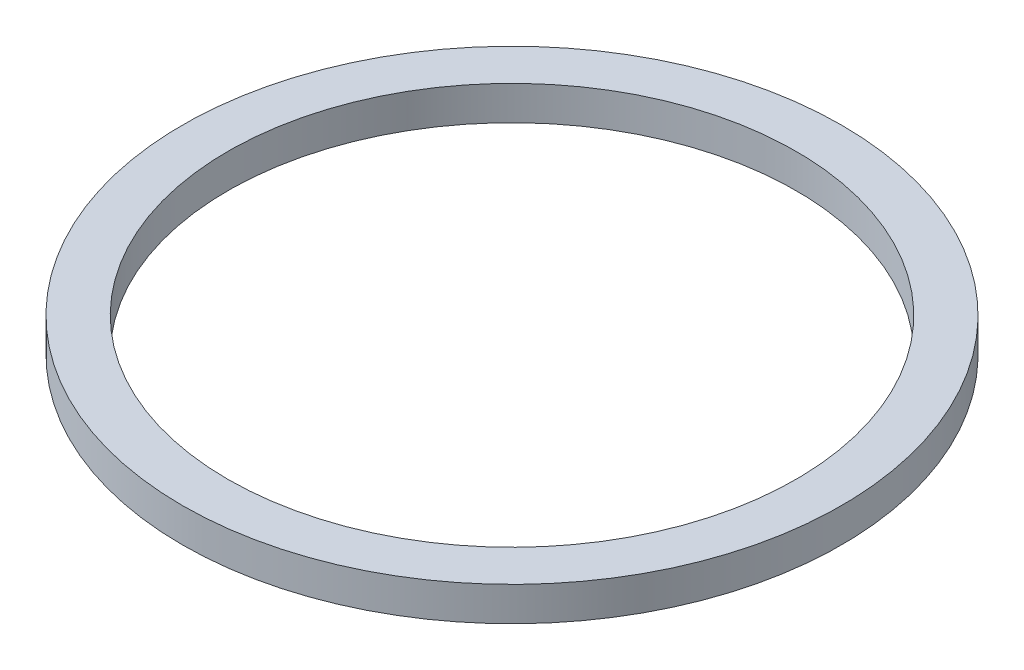
from build123d import *

# Parameters (mm, degrees)
SKETCH_1_R      = 29
SKETCH_1_R_2    = 25
EXTRUDE_1_DEPTH = 3


with BuildPart() as part:
    # 草图1 → 凸台-拉伸1 (new body)
    with BuildSketch(Plane(origin=(0, 0, 0), x_dir=(1, 0, 0), z_dir=(0, 1, 0))):
        with Locations(Location((0, 0, 0), (0, 0, 270))):
            Circle(SKETCH_1_R)
        with Locations(Location((0, 0, 0), (0, 0, 270))):
            Circle(SKETCH_1_R_2, mode=Mode.SUBTRACT)
    extrude(amount=EXTRUDE_1_DEPTH)


solid = part.part
